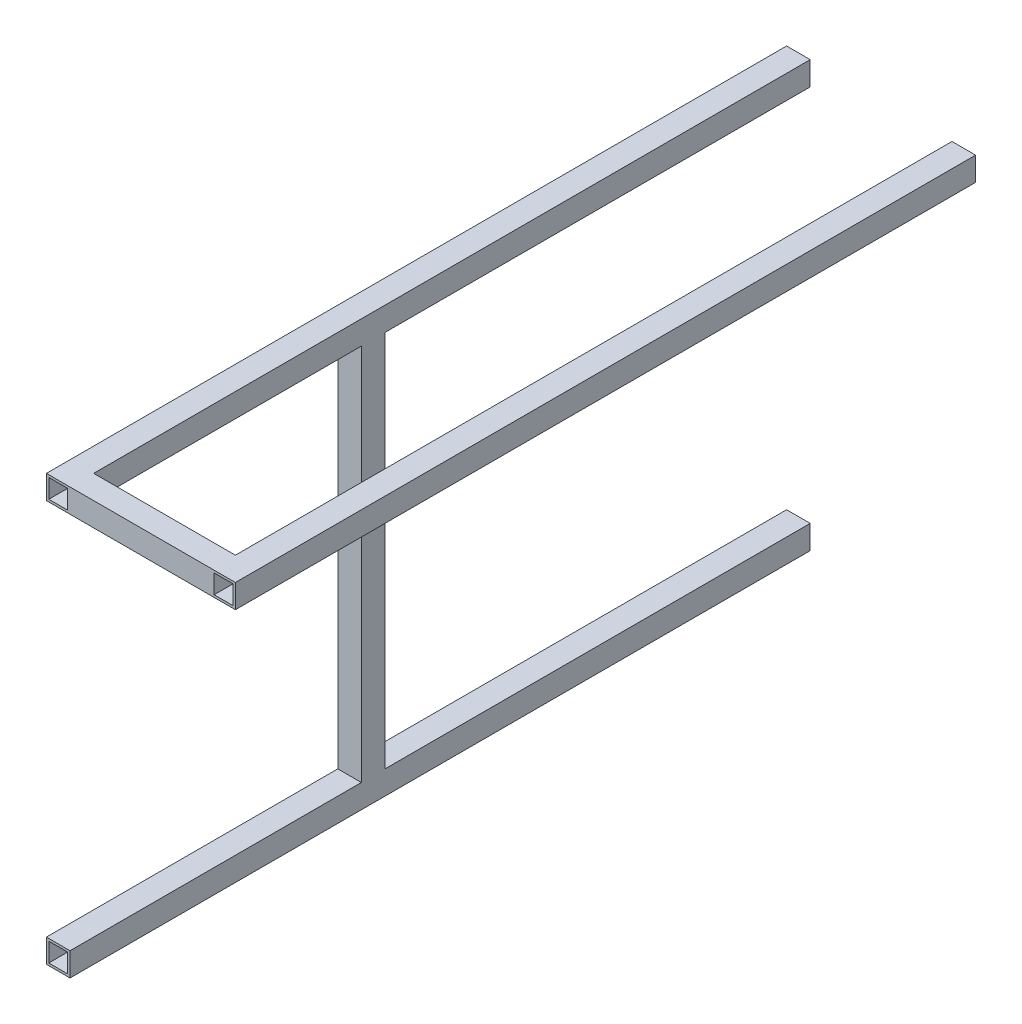
SolidWorks part; units mm, degrees
ref_plane "前视基准面" through (0, 0, 0) normal (0, 0, 1) x (1, 0, 0)
ref_plane "上视基准面" through (0, 0, 0) normal (0, 1, 0) x (1, 0, 0)
ref_plane "右视基准面" through (0, 0, 0) normal (1, 0, 0) x (0, 0, -1)
sketch "草图1" plane through (0, 0, 0) normal (0, 0, 1) x (1, 0, 0)
  line L0 (0, 0) -> (0, 30)
  line L1 (0, 30) -> (30, 30)
  line L2 (30, 30) -> (30, 0)
  line L3 (30, 0) -> (0, 0)
  line L4 (3, 3) -> (3, 27)
  line L5 (3, 27) -> (27, 27)
  line L6 (27, 27) -> (27, 3)
  line L7 (27, 3) -> (3, 3)
  line L8 (0, 30) -> (240, 30)
  line L9 (0, 30) -> (0, -510)
  line L18 (213, 3) -> (213, 27)
  line L19 (210, 0) -> (210, 30)
  line L20 (240, 30) -> (240, 0)
  line L21 (237, 3) -> (213, 3)
  line L22 (210, 30) -> (240, 30)
  line L23 (240, 0) -> (210, 0)
  line L24 (213, 27) -> (237, 27)
  line L25 (237, 27) -> (237, 3)
  line L34 (3, -507) -> (3, -483)
  line L35 (0, -510) -> (0, -480)
  line L36 (30, -480) -> (30, -510)
  line L37 (27, -507) -> (3, -507)
  line L38 (27, -483) -> (27, -507)
  line L39 (30, -510) -> (0, -510)
  line L40 (0, -480) -> (30, -480)
  line L41 (3, -483) -> (27, -483)
  dimension "D1" = 3
extrude "凸台-拉伸1" add sketch "草图1" along normal blind 940 contours L3 L2 L1 L0 L6 L7 L4 L5 | L23 L20 L8 L19 L24 L25 L21 L18 | L40 L9 L39 L36 L34 L41 L38 L37
sketch "草图3" plane through (0, 0, 0) normal (0, -1, 0) x (1, 0, 0)
  line L0 (0, 370) -> (0, 400)
  line L1 (0, 940) -> (0, 0) construction
  line L2 (0, 400) -> (30, 400)
  line L3 (30, 940) -> (30, 0) construction
  line L4 (30, 400) -> (30, 370)
  line L5 (30, 370) -> (0, 370)
  line L6 (0, 370) -> (0, 400)
  line L7 (0, 400) -> (0, 370)
  line L8 (3, 370) -> (3, 400) construction
  line L9 (3, 397) -> (27, 397)
  line L10 (27, 397) -> (27, 373)
  line L11 (27, 373) -> (3, 373)
  line L12 (3, 373) -> (3, 397)
  line L13 (0, 397) -> (27, 397) construction
  line L14 (27, 373) -> (0, 373) construction
  line M2 (30, 0) -> (30, 940)
  line M4 (0, 940) -> (0, 0)
  dimension "D1" = 3
extrude "凸台-拉伸2" add sketch "草图3" along normal blind 480 contours L5 L2 L11 L12 L9 L10 M2 M4
sketch "草图4" plane through (0, 0, 0) normal (-1, 0, 0) x (0, 0, 1)
  line L0 (370, 0) -> (400, 0)
  line L1 (400, 0) -> (400, -480)
  line L2 (400, -480) -> (370, -480)
  line L3 (370, -480) -> (370, 0)
extrude "切除-拉伸1" cut sketch "草图4" against normal blind 37
sketch "草图5" plane through (0, 0, 0) normal (-1, 0, 0) x (0, 0, 1)
  line L0 (0, 0) -> (540, 0)
  line L1 (940, 0) -> (0, 0) construction
  line L2 (540, 0) -> (540, -480)
  line L3 (940, -480) -> (0, -480) construction
  line L4 (540, -480) -> (570, -480)
  line L5 (570, -480) -> (570, 0)
  line L6 (570, 0) -> (540, 0)
  line M1 (0, 0) -> (940, 0)
extrude "凸台-拉伸3" add sketch "草图5" against normal blind 30 contours L4 L5 L2 M1
sketch "草图6" plane through (210, 0, 0) normal (-1, 0, 0) x (0, 0, 1)
  line L0 (940, 30) -> (910, 30)
  line L1 (940, 30) -> (0, 30) construction
  line L2 (910, 30) -> (910, 0)
  line L3 (940, 0) -> (0, 0) construction
  line L4 (910, 0) -> (940, 0)
  line L5 (940, 0) -> (940, 30)
extrude "凸台-拉伸4" add sketch "草图6" along normal blind 180
